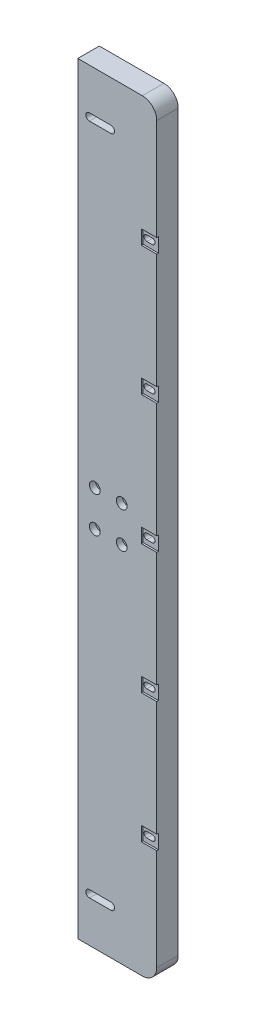
SolidWorks part; units mm, degrees
ref_plane "前视基准面" through (0, 0, 0) normal (0, 0, 1) x (1, 0, 0)
ref_plane "上视基准面" through (0, 0, 0) normal (0, 1, 0) x (1, 0, 0)
ref_plane "右视基准面" through (0, 0, 0) normal (1, 0, 0) x (0, 0, -1)
sketch "草图1" plane through (0, 0, 0) normal (0, 0, 1) x (1, 0, 0)
  line L1 (22, 212.5) -> (-22, 212.5)
  line L2 (22, 212.5) -> (22, -212.5)
  line L3 (22, -212.5) -> (-22, -212.5)
  line L4 (-22, 212.5) -> (-22, -212.5)
  line L5 (22, 212.5) -> (-22, -212.5) construction
  line L6 (22, -212.5) -> (-22, 212.5) construction
  point P0 (0, 0)
  dimension "D1" = 44
  dimension "D2" = 425
extrude "凸台-拉伸1" add sketch "草图1" along normal blind 12
fillet "圆角1" radius 8 2 edges at (22, 212.5, 6) (22, -212.5, 6)
sketch "草图3" plane through (0, 0, 0) normal (0, 0, -1) x (-1, 0, 0)
  line L0 (15.5, 187.5) -> (3.5, 187.5) construction
  line L1 (15.5, 183.5) -> (3.5, 183.5)
  line L2 (15.5, 191.5) -> (3.5, 191.5)
  line L3 (-14, 212.5) -> (22, 212.5) construction
  line L4 (22, 212.5) -> (22, -212.5) construction
  line L5 (41.3054, 0) -> (-37.934, 0) construction
  line L6 (15.5, -187.5) -> (3.5, -187.5) construction
  line L7 (15.5, -183.5) -> (3.5, -183.5)
  line L8 (15.5, -191.5) -> (3.5, -191.5)
  arc A0 (15.5, 183.5) -> (15.5, 191.5) centre (15.5, 187.5) ccw
  arc A1 (3.5, 191.5) -> (3.5, 183.5) centre (3.5, 187.5) ccw
  arc A2 (15.5, -183.5) -> (15.5, -191.5) centre (15.5, -187.5) cw
  arc A3 (3.5, -191.5) -> (3.5, -183.5) centre (3.5, -187.5) cw
  point P2 (9.5, 187.5)
  point P16 (9.5, -187.5)
  dimension "D1" = 4
  dimension "D2" = 12
  dimension "D3" = 25
  dimension "D4" = 6.5
extrude "切除-拉伸1" cut sketch "草图3" against normal blind 6
sketch "草图4" plane through (0, 0, 0) normal (0, 0, -1) x (-1, 0, 0)
  line L0 (3.5, 187.5) -> (15.5, 187.5) construction
  line L1 (3.5, 189.5) -> (15.5, 189.5)
  line L2 (3.5, 185.5) -> (15.5, 185.5)
  line L3 (-37.5197, 0) -> (61.185, 0) construction
  line L4 (3.5, -187.5) -> (15.5, -187.5) construction
  line L5 (3.5, -189.5) -> (15.5, -189.5)
  line L6 (3.5, -185.5) -> (15.5, -185.5)
  arc A0 (3.5, 189.5) -> (3.5, 185.5) centre (3.5, 187.5) ccw
  arc A1 (15.5, 185.5) -> (15.5, 189.5) centre (15.5, 187.5) ccw
  arc A2 (3.5, -189.5) -> (3.5, -185.5) centre (3.5, -187.5) cw
  arc A3 (15.5, -185.5) -> (15.5, -189.5) centre (15.5, -187.5) cw
  point P4 (9.5, 187.5)
  point P14 (9.5, -187.5)
  dimension "D1" = 2
extrude "切除-拉伸2" cut sketch "草图4" against normal through all
sketch "草图5" plane through (0, 0, 12) normal (0, 0, 1) x (1, 0, 0)
  line L0 (22, -204.5) -> (22, 204.5) construction
  line L1 (22, 148) -> (13.5, 148)
  line L2 (22, 148) -> (22, 140)
  line L3 (22, 140) -> (13.5, 140)
  line L4 (13.5, 148) -> (13.5, 140)
  line L5 (14, 212.5) -> (-22, 212.5) construction
  line L6 (13.5, 76) -> (13.5, 68)
  line L7 (22, 68) -> (13.5, 68)
  line L8 (22, 76) -> (22, 68)
  line L9 (22, 76) -> (13.5, 76)
  line L10 (13.5, 4) -> (13.5, -4)
  line L11 (22, -4) -> (13.5, -4)
  line L12 (22, 4) -> (22, -4)
  line L13 (22, 4) -> (13.5, 4)
  line L14 (13.5, -68) -> (13.5, -76)
  line L15 (22, -76) -> (13.5, -76)
  line L16 (22, -68) -> (22, -76)
  line L17 (22, -68) -> (13.5, -68)
  line L18 (13.5, -140) -> (13.5, -148)
  line L19 (22, -148) -> (13.5, -148)
  line L20 (22, -140) -> (22, -148)
  line L21 (22, -140) -> (13.5, -140)
  dimension "D1" = 64.5
  dimension "D2" = 8
  dimension "D3" = 8.5
extrude "切除-拉伸3" cut sketch "草图5" against normal blind 1
sketch "草图6" plane through (0, 0, 0) normal (0, 0, -1) x (-1, 0, 0)
  line L0 (-18.5, 144) -> (-15.5, 144) construction
  line L1 (-18.5, 147) -> (-15.5, 147)
  line L2 (-18.5, 141) -> (-15.5, 141)
  line L3 (-22, -204.5) -> (-22, 204.5) construction
  line L4 (-14, 212.5) -> (22, 212.5) construction
  arc A0 (-18.5, 147) -> (-18.5, 141) centre (-18.5, 144) ccw
  arc A1 (-15.5, 141) -> (-15.5, 147) centre (-15.5, 144) ccw
  point P2 (-17, 144)
  dimension "D2" = 3
  dimension "D1" = 3.5
  dimension "D3" = 3
  dimension "D4" = 68.5
extrude "切除-拉伸4" cut sketch "草图6" against normal blind 4
sketch "草图7" plane through (0, 0, 4) normal (0, 0, -1) x (-1, 0, 0)
  line L0 (-18.5, 144) -> (-15.5, 144) construction
  line L1 (-18.5, 145.6) -> (-15.5, 145.6)
  line L2 (-18.5, 142.4) -> (-15.5, 142.4)
  arc A0 (-18.5, 145.6) -> (-18.5, 142.4) centre (-18.5, 144) ccw
  arc A1 (-15.5, 142.4) -> (-15.5, 145.6) centre (-15.5, 144) ccw
  point P4 (-17, 144)
  dimension "D1" = 1.6
extrude "切除-拉伸5" cut sketch "草图7" against normal through all
pattern_linear "阵列(线性)1" count 5 spacing 72 along (0, -1, 0) of "切除-拉伸4", "切除-拉伸5"
hole_wizard "打孔尺寸根据内六角圆柱头螺钉的类型1" positions "草图9" profile "草图8" counterbore size "M3" standard "Gb" end condition through all
sketch "草图9" plane through (0, 0, 12) normal (0, 0, 1) x (1, 0, 0)
  point P0 (2.5, 10)
  point P3 (-12.5, 10)
  point P6 (2.5, -10)
  point P9 (-12.5, -10)
sketch "草图8" plane through (2.5, 10, 12) normal (1, 0, 0) x (0, -1, 0)
  line L0 (0, 0) -> (0, 12)
  line L1 (0, 12) -> (1.7, 12)
  line L3 (1.7, 12) -> (1.7, 3.4)
  line L4 (1.7, 3.4) -> (3, 3.4)
  line L5 (3, 3.4) -> (3, 0)
  line L7 (3, 0) -> (0, 0)
  line L11 (0, -6.35) -> (0, 107.95) construction
  dimension "通孔孔直径" = 3.4
  dimension "通孔孔深度" = 12
  dimension "柱形沉头孔直径" = 6
  dimension "柱形沉头孔深度" = 3.4
